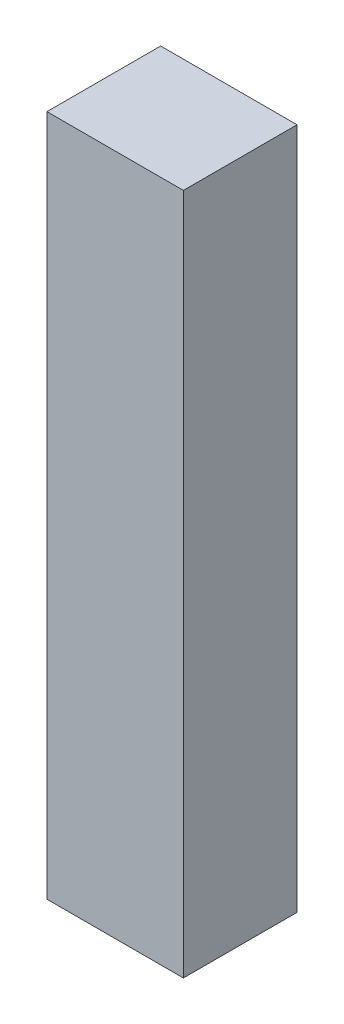
from build123d import *

# Parameters (mm, degrees)
SKETCH1_W           = 12
SKETCH1_H           = 60
BOSS_EXTRUDE1_DEPTH = 10


with BuildPart() as part:
    # Sketch1 → Boss-Extrude1 (new body)
    with BuildSketch(Plane.XY):
        with Locations((-37.66548583, 8.769230769)):
            Rectangle(SKETCH1_W, SKETCH1_H)
    extrude(amount=BOSS_EXTRUDE1_DEPTH)


solid = part.part
